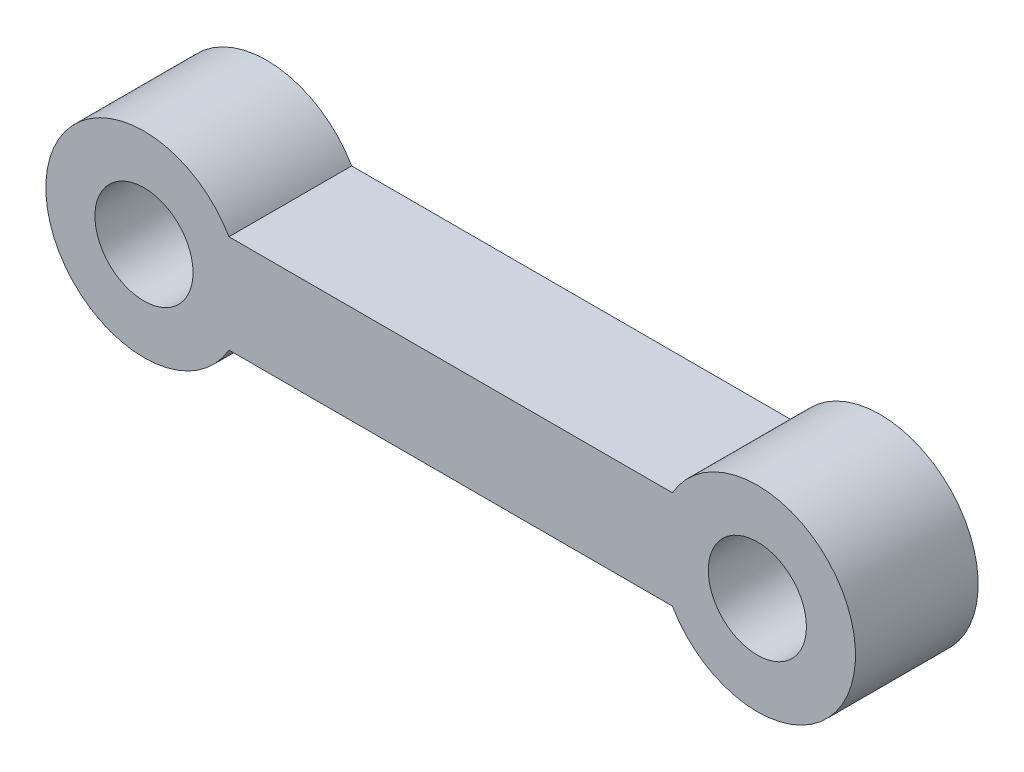
from build123d import *

# Parameters (mm, degrees)
SKETCH1_R           = 4
BOSS_EXTRUDE1_DEPTH = 10


with BuildPart() as part:
    # Sketch1 → Boss-Extrude1 (new body)
    with BuildSketch(Plane.XY):
        with BuildLine():
            Line((6.92820323, -4), (43.07179677, -4))
            ThreePointArc((43.07179677, -4), (58, 0), (43.07179677, 4))
            Line((43.07179677, 4), (6.92820323, 4))
            ThreePointArc((6.92820323, 4), (-8, 0), (6.92820323, -4))
        make_face()
        Circle(SKETCH1_R, mode=Mode.SUBTRACT)
        with Locations((50, 0)):
            Circle(SKETCH1_R, mode=Mode.SUBTRACT)
    extrude(amount=BOSS_EXTRUDE1_DEPTH)


solid = part.part
